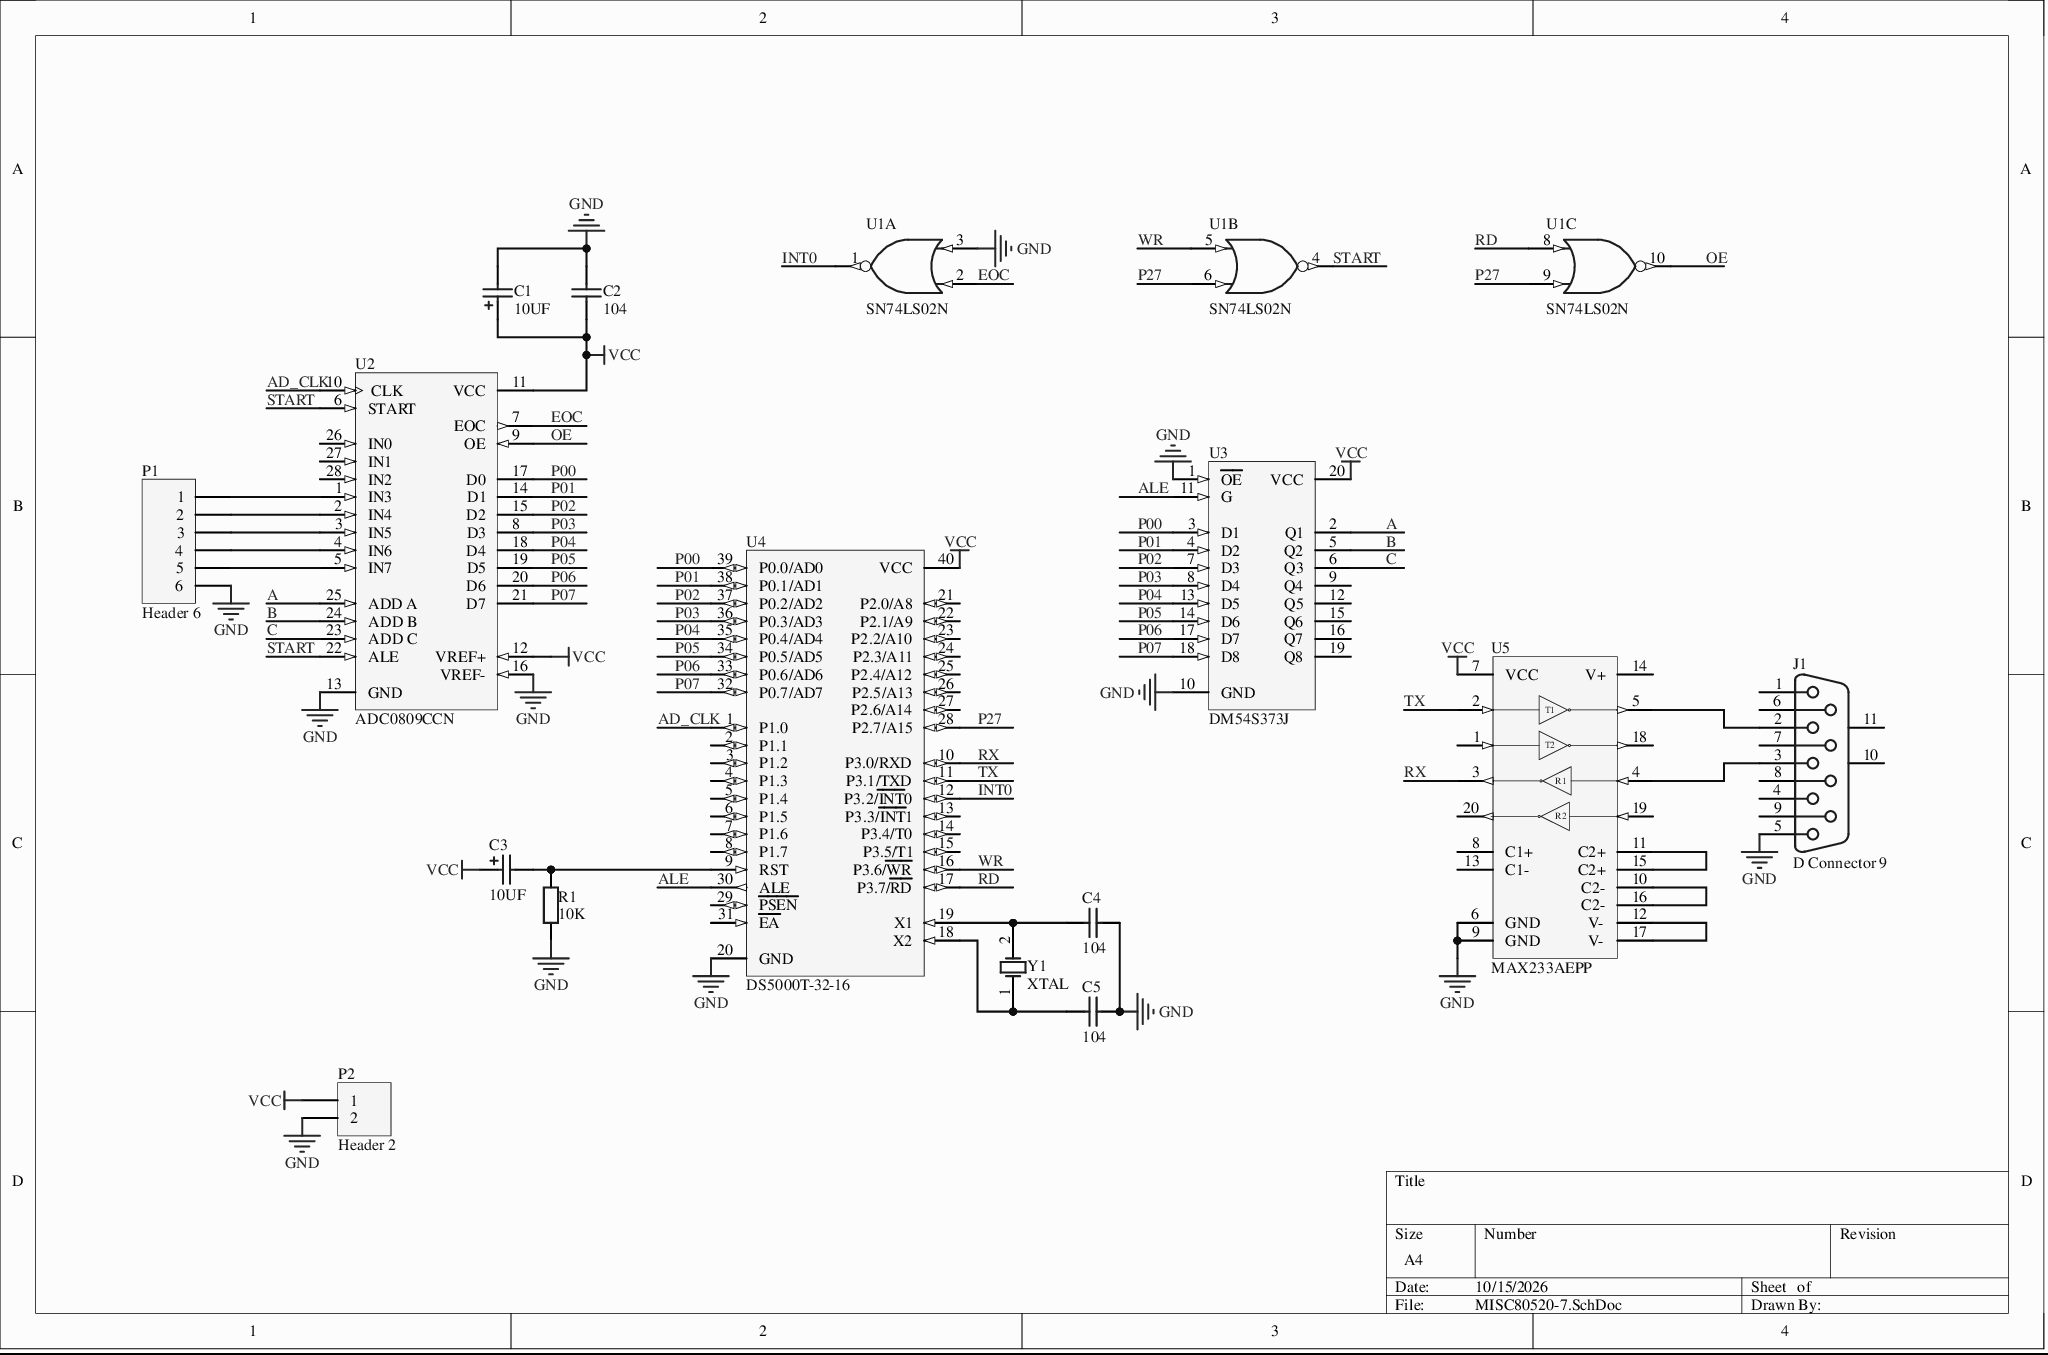
[diagram p0: MISC80520-7.SchDoc]
# Altium project MISC80520-3.PrjPcb
1 sheet, 15 parts. Net scope: global (net labels, ports and power ports of the same name join across sheets).
Board file: MISC80520.PcbDoc

## Sheet MISC80520-7.SchDoc
size A4

### Parts
C1  10UF  [POLAR0.8]
C2  104  [RAD-0.1]
C3  10UF  [POLAR0.8]
C4  104  [RAD-0.1]
C5  104  [RAD-0.1]
J1  D Connector 9  [DSUB1.385-2H9]
P1  Header 6  [HDR1X6]
P2  Header 2  [HDR1X2]
R1  10K  [AXIAL-0.4]
U1  SN74LS02N  [N014]  (parts A,B,C of 4)
U2  ADC0809CCN  [N28B]
U3  DM54S373J  [J20A]
U4  DS5000T-32-16  [ENDIP40A]
U5  MAX233AEPP  [PP20]
Y1  XTAL  [R38]

### Nets
GND: C1.2 C2.2 C4.1 C5.2 J1.5 P1.6 P2.2 R1.1 U1.3(B) U1.7(GND) U2.13(GND) U2.16(VREF-) U3.1(~{OE}) U3.10(GND) U4.20(GND) U5.6(GND) U5.9(GND)
VCC: C1.1 C2.1 C3.1 P2.1 U1.14(VCC) U2.11(VCC) U2.12(VREF+) U3.20(VCC) U4.40(VCC) U5.7(VCC)
A: U2.25(ADD_A) U3.2(Q1)
AD_CLK: U2.10(CLK) U4.1(P1.0)
ALE: U3.11(G) U4.30(ALE)
B: U2.24(ADD_B) U3.5(Q2)
C: U2.23(ADD_C) U3.6(Q3)
EOC: U1.2(A) U2.7(EOC)
INT0: U1.1(Y) U4.12(P3.2/~{INT}0)
OE: U1.10(Y) U2.9(OE)
P00: U2.17(D0) U3.3(D1) U4.39(P0.0/AD0)
P01: U2.14(D1) U3.4(D2) U4.38(P0.1/AD1)
P02: U2.15(D2) U3.7(D3) U4.37(P0.2/AD2)
P03: U2.8(D3) U3.8(D4) U4.36(P0.3/AD3)
P04: U2.18(D4) U3.13(D5) U4.35(P0.4/AD4)
P05: U2.19(D5) U3.14(D6) U4.34(P0.5/AD5)
P06: U2.20(D6) U3.17(D7) U4.33(P0.6/AD6)
P07: U2.21(D7) U3.18(D8) U4.32(P0.7/AD7)
P27: U1.6(B) U1.9(B) U4.28(P2.7/A15)
RD: U1.8(A) U4.17(P3.7/~{RD})
RX: U4.10(P3.0/RXD) U5.3(R1OUT)
START: U1.4(Y) U2.6(START) U2.22(ALE)
TX: U4.11(P3.1/TXD) U5.2(T1IN)
WR: U1.5(A) U4.16(P3.6/~{WR})
NetC3_2: C3.2 R1.2 U4.9(RST)
NetC4_2: C4.2 U4.19(X1) Y1.2(OSC2)
NetC5_1: C5.1 U4.18(X2) Y1.1(OSC1)
NetJ1_2: J1.2 U5.5(T1OUT)
NetJ1_3: J1.3 U5.4(R1IN)
NetP1_1: P1.1 U2.1(IN3)
NetP1_2: P1.2 U2.2(IN4)
NetP1_3: P1.3 U2.3(IN5)
NetP1_4: P1.4 U2.4(IN6)
NetP1_5: P1.5 U2.5(IN7)
NetU5_10: U5.10(C2-) U5.16(C2-)
NetU5_11: U5.11(C2+) U5.15(C2+)
NetU5_12: U5.12(V-) U5.17(V-)

Not connected (* = marked no-connect by the designer): J1 1 4 6 7 8 9 10(MH1) 11(MH2); U2 26(IN0) 27(IN1) 28(IN2); U3 9(Q4) 12(Q5) 15(Q6) 16(Q7) 19(Q8); U4 2(P1.1) 3(P1.2) 4(P1.3) 5(P1.4) 6(P1.5) 7(P1.6) 8(P1.7) 13(P3.3/~{INT}1) 14(P3.4/T0) 15(P3.5/T1) 21(P2.0/A8) 22(P2.1/A9) 23(P2.2/A10) 24(P2.3/A11) 25(P2.4/A12) 26(P2.5/A13) 27(P2.6/A14) 29(~{PSEN}) 31(~{EA}); U5 1(T2IN) 8(C1+) 13(C1-) 14(V+) 18(T2OUT) 19(R2IN) 20(R2OUT)

### Library data of the parts
C1 C3 = Cap Pol2: Polarized Capacitor (Axial); Value: 100pF; Published: 8-Jun-2000; LatestRevisionDate: 17-Jul-2002; LatestRevisionNote: Re-released for DXP Platform.; PackageReference: POLAR0.8; PackageDescription: Polarized Capacitor; 2 Leads; Publisher: Altium Limited
C2 C4 C5 = Cap: Capacitor; Value: 100pF; Published: 8-Jun-2000; LatestRevisionDate: 17-Jul-2002; LatestRevisionNote: Re-released for DXP Platform.; PackageReference: RAD-0.3; PackageDescription: Radial Cap, Thru-Hole; 2 Leads; 0.3 in Pin Spacing; Publisher: Altium Limited
J1 = D Connector 9: Receptacle Assembly, 9 Position, Right Angle; PackageDocument: O; Positions: 9; Published: 15-Jun-2001; LatestRevisionDate: 17-Jul-2002; LatestRevisionNote: Re-released for DXP Platform.; DatasheetDocument: 1-Sep-1999; PackageReference: 788750; Orientation: Right Angle; Gender: Receptacle; Publisher: Altium Limited
P1 = Header 6: Header, 6-Pin; LatestRevisionDate: 17-Jul-2002; LatestRevisionNote: Re-released for DXP Platform.; Publisher: Altium Limited
P2 = Header 2: Header, 2-Pin; LatestRevisionDate: 17-Jul-2002; LatestRevisionNote: Re-released for DXP Platform.; Publisher: Altium Limited
R1 = Res2: Resistor; Value: 1K; Published: 8-Jun-2000; LatestRevisionDate: 17-Jul-2002; LatestRevisionNote: Re-released for DXP Platform.; PackageReference: AXIAL-0.4; PackageDescription: Axial Device, Thru-Hole; 2 Leads; 0.4 in Pin Spacing; Publisher: Altium Limited
U1 = SN74LS02N: Quadruple 2-Input Positive-NOR Gate; Package Information: Latest Revision: Oct-1995; Published: 8-Jun-2000; Revision: 17-Jul-2002: Re-released for DXP Platform.; Datasheet: Latest Revision: Mar-1988; Package Reference: N014; Publisher: Altium Limited
U2 = ADC0809CCN: 8-Bit µP-Compatible A/D Converter with 8-Channel Multiplexer; Package Information: Latest Revision: 2000; Published: 15-Apr-2002; Datasheet: Latest Revision: Oct-1999; Package Reference: N28B; Publisher: Altium Limited
U3 = DM54S373J: Octal D-Type Transparent Latch and Edge-Triggered Flip-Flop; Package Information: Latest Revision: 2000; Code - JEDEC: MS-015-AE; Published: 15-Apr-2002; Datasheet: Latest Revision: 1989; Package Reference: J20A; Publisher: Altium Limited
U4 = DS5000T-32-16: Soft Microcontroller; Published: 13-Oct-2000; Revision: 17-Jul-2002: PCB footprint, 'DIP-P40/X1.1' replaced; Re-released for DXP Platform.; Datasheet: Latest Revision: 21-Apr-1993; Package Reference: ENDIP40A; Publisher: Altium Limited
U5 = MAX233AEPP: +5V-Powered, Multichannel RS-232 Driver/Receiver; Package Information: Latest Revision: RevB, 21-0043; Code - JEDEC: MS-001-AE; Published: 16-Jan-2001; Revision: 17-Jul-2002: Re-released for DXP Platform.; Datasheet: Latest Revision: Nov-1997; Package Reference: PP20; Publisher: Altium Limited
Y1 = XTAL: Crystal Oscillator; Published: 8-Jun-2000; LatestRevisionDate: 17-Jul-2002; LatestRevisionNote: Re-released for DXP Platform.; PackageReference: R38; PackageDescription: Crystal, Thru-Hole; 2 Leads; Body 3.1 x 8.2 mm (Dia.xH); Publisher: Altium Limited